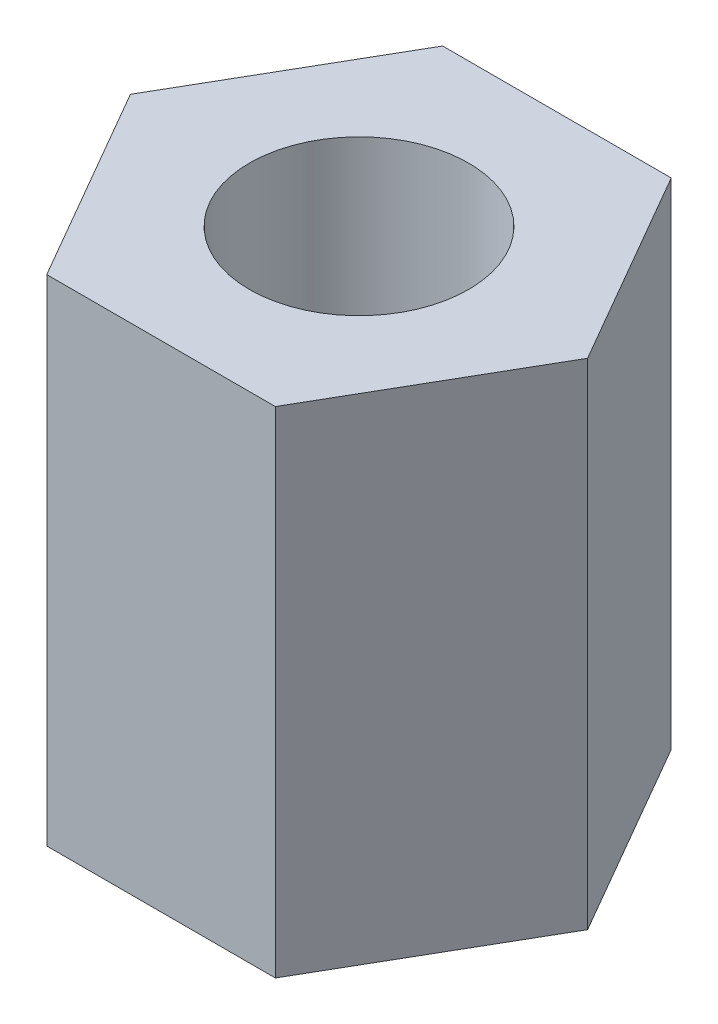
SolidWorks part; units mm, degrees
material "尼龙 101"
ref_plane "前视基准面" through (0, 0, 0) normal (0, 0, 1) x (1, 0, 0)
ref_plane "上视基准面" through (0, 0, 0) normal (0, 1, 0) x (1, 0, 0)
ref_plane "右视基准面" through (0, 0, 0) normal (1, 0, 0) x (0, 0, -1)
other "Configuration Table"
sketch "草图1" plane through (0, 0, 0) normal (0, 1, 0) x (1, 0, 0)
  line L1 (1.6166, -2.8) -> (3.2332, 0)
  line L2 (3.2332, 0) -> (1.6166, 2.8)
  line L3 (1.6166, 2.8) -> (-1.6166, 2.8)
  line L4 (-1.6166, 2.8) -> (-3.2332, 0)
  line L5 (-3.2332, 0) -> (-1.6166, -2.8)
  line L6 (-1.6166, -2.8) -> (1.6166, -2.8)
  circle A0 centre (0, 0) radius 2.8 construction
  circle A1 centre (0, 0) radius 1.55
  dimension "D1" = 5.6
  dimension "D2" = 3.1
extrude "凸台-拉伸1" add sketch "草图1" along normal blind 7
